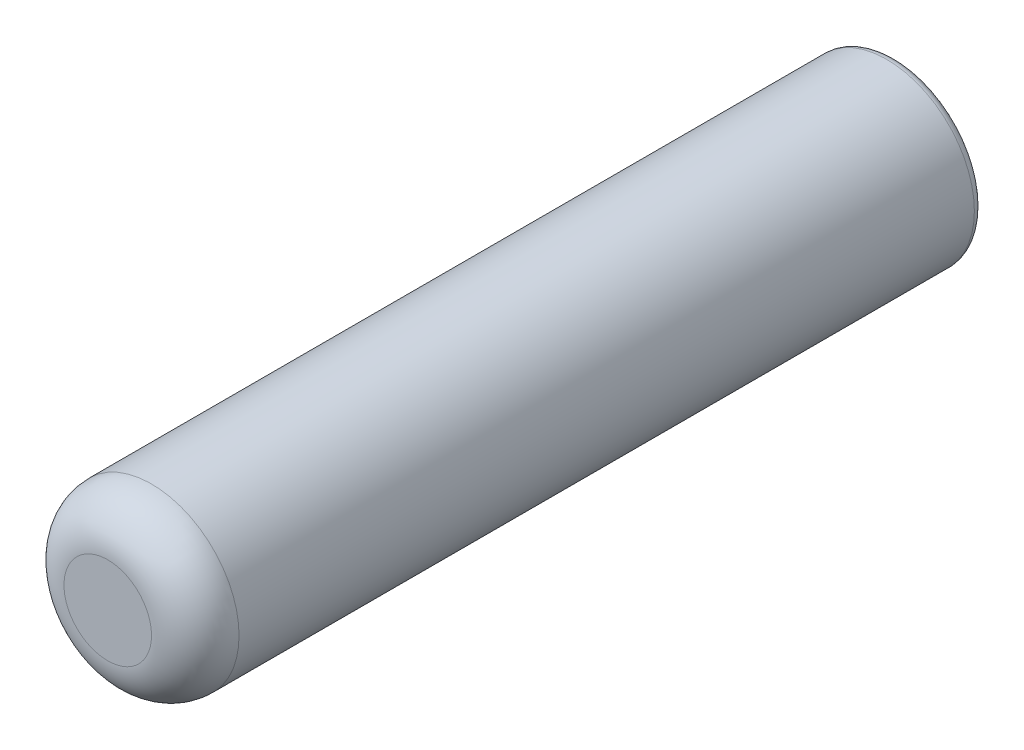
from build123d import *

# Parameters (mm, degrees)
SKETCH1_R           = 1
BOSS_EXTRUDE1_DEPTH = 9
FILLET1_R           = 0.5
FILLET2_R           = 0.1


with BuildPart() as part:
    # Sketch1 → Boss-Extrude1 (new body)
    with BuildSketch(Plane.XY):
        Circle(SKETCH1_R)
    extrude(amount=BOSS_EXTRUDE1_DEPTH)

    # Fillet1
    fillet1_edges = [part.edges().sort_by_distance(p)[0] for p in [
        (-1, 0, 9),
    ]]
    fillet(fillet1_edges, radius=FILLET1_R)

    # Fillet2
    fillet2_edges = [part.edges().sort_by_distance(p)[0] for p in [
        (-1, 0, 0),
    ]]
    fillet(fillet2_edges, radius=FILLET2_R)


solid = part.part
